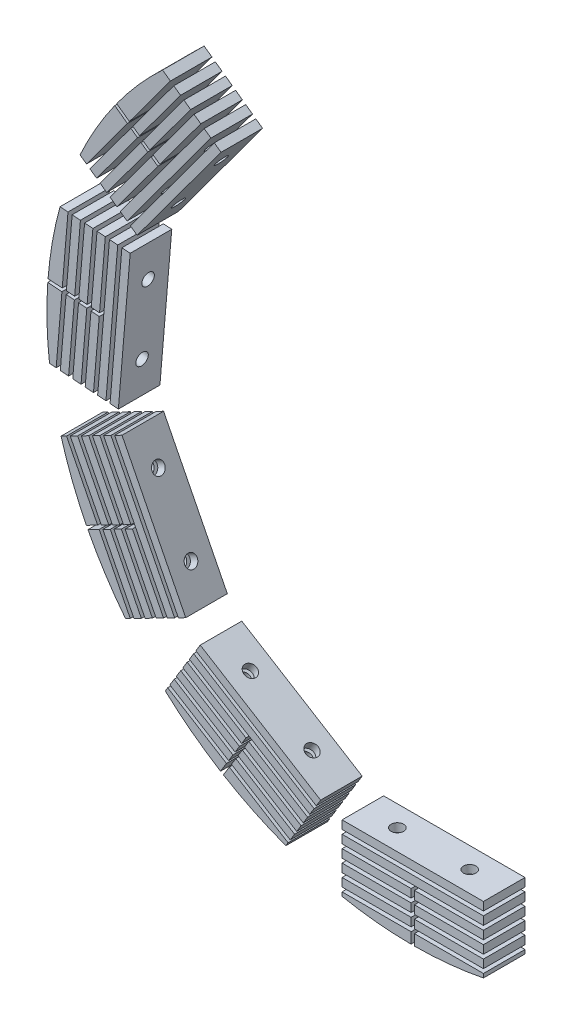
from build123d import *

# Parameters (mm, degrees)
EXTRUDE_1_DEPTH      = 25
EXTRUDE_1_2_DEPTH    = 25
EXTRUDE_1_3_DEPTH    = 25
EXTRUDE_1_4_DEPTH    = 25
EXTRUDE_1_5_DEPTH    = 25
EXTRUDE_1_6_DEPTH    = 25
EXTRUDE_1_7_DEPTH    = 25
EXTRUDE_1_8_DEPTH    = 25
EXTRUDE_1_9_DEPTH    = 25
EXTRUDE_1_10_DEPTH   = 25
SKETCH_3_W           = 195
SKETCH_3_H           = 5
CUT_EXTRUDE_2_DEPTH  = 50
SKETCH_9_R           = 7.5
CUT_EXTRUDE_5_DEPTH  = 25
SKETCH_10_R          = 7.5
CUT_EXTRUDE_6_DEPTH  = 25
SKETCH_11_R          = 7.5
CUT_EXTRUDE_7_DEPTH  = 25
SKETCH_12_R          = 7.5
CUT_EXTRUDE_8_DEPTH  = 25
SKETCH_13_R          = 7.5
CUT_EXTRUDE_9_DEPTH  = 25
SKETCH_15_W          = 182.108507318
SKETCH_15_H          = 36.421701464
CUT_EXTRUDE_13_DEPTH = 146
SKETCH_16_R          = 12.379446908
SKETCH_16_R_2        = 10.572142033
SKETCH_16_R_3        = 6.534828031
SKETCH_16_R_4        = 5.127216656
CUT_EXTRUDE_14_DEPTH = 146
SKETCH_17_W          = 4
SKETCH_17_H          = 10
EXTRUDE_2_DEPTH      = 50


with BuildPart() as part:
    # 草图2 → 凸台-拉伸1 (new, symmetric)
    with BuildSketch(Plane.XY):
        with BuildLine():
            Line((-85, -337), (-85, -431.711709362))
            ThreePointArc((-85, -431.711709362), (-43.69674025, -437.824844991), (-2, -439.995454522))
            Line((-2, -439.995454522), (-2, -337))
            Line((-2, -337), (-85, -337))
        make_face()
    extrude(amount=EXTRUDE_1_DEPTH, both=True)


with BuildPart() as body_2:
    # 草图2 → Extrude 1 2 (new, symmetric)
    with BuildSketch(Plane.XY):
        with BuildLine():
            Line((85, -337), (85, -431.711709362))
            ThreePointArc((85, -431.711709362), (43.69674025, -437.824844991), (2, -439.995454522))
            Line((2, -439.995454522), (2, -337))
            Line((2, -337), (85, -337))
        make_face()
    extrude(amount=EXTRUDE_1_2_DEPTH, both=True)


with BuildPart() as body_3:
    # 草图2 → Extrude 1 3 (new, symmetric)
    with BuildSketch(Plane.XY):
        with BuildLine():
            Line((-248.253388478, -243.237034823), (-177.430245302, -286.516156703))
            Line((-177.430245302, -286.516156703), (-231.135701078, -374.401238896))
            ThreePointArc((-231.135701078, -374.401238896), (-265.583317105, -350.806929344), (-297.639407911, -324.053672805))
            Line((-297.639407911, -324.053672805), (-248.253388478, -243.237034823))
        make_face()
    extrude(amount=EXTRUDE_1_3_DEPTH, both=True)


with BuildPart() as body_4:
    # 草图2 → Extrude 1 4 (new, symmetric)
    with BuildSketch(Plane.XY):
        with BuildLine():
            Line((-174.017081776, -288.601897517), (-227.722537551, -376.48697971))
            ThreePointArc((-227.722537551, -376.48697971), (-191.01125708, -396.376966622), (-152.579958034, -412.697657379))
            Line((-152.579958034, -412.697657379), (-103.1939386, -331.881019397))
            Line((-103.1939386, -331.881019397), (-174.017081776, -288.601897517))
        make_face()
    extrude(amount=EXTRUDE_1_4_DEPTH, both=True)


with BuildPart() as body_5:
    # 草图2 → Extrude 1 5 (new, symmetric)
    with BuildSketch(Plane.XY):
        with BuildLine():
            Line((-338.664705444, -78.103887779), (-300.799220884, -151.96324791))
            Line((-300.799220884, -151.96324791), (-392.451972299, -198.950871922))
            ThreePointArc((-392.451972299, -198.950871922), (-409.542905348, -160.855863054), (-422.94598557, -121.312378966))
            Line((-422.94598557, -121.312378966), (-338.664705444, -78.103887779))
        make_face()
    extrude(amount=EXTRUDE_1_5_DEPTH, both=True)


with BuildPart() as body_6:
    # 草图2 → Extrude 1 6 (new, symmetric)
    with BuildSketch(Plane.XY):
        with BuildLine():
            Line((-298.974378255, -155.522735146), (-390.62712967, -202.510359157))
            ThreePointArc((-390.62712967, -202.510359157), (-369.673068161, -238.624857624), (-345.39017382, -272.590586464))
            Line((-345.39017382, -272.590586464), (-261.108893694, -229.382095277))
            Line((-261.108893694, -229.382095277), (-298.974378255, -155.522735146))
        make_face()
    extrude(amount=EXTRUDE_1_6_DEPTH, both=True)


with BuildPart() as body_7:
    # 草图2 → Extrude 1 7 (new, symmetric)
    with BuildSketch(Plane.XY):
        with BuildLine():
            Line((-329.705621695, 109.946364299), (-335.908219463, 27.178449133))
            Line((-335.908219463, 27.178449133), (-438.615677805, 34.875309088))
            ThreePointArc((-438.615677805, 34.875309088), (-433.335136437, 76.293246942), (-424.152497908, 117.024179203))
            Line((-424.152497908, 117.024179203), (-329.705621695, 109.946364299))
        make_face()
    extrude(amount=EXTRUDE_1_7_DEPTH, both=True)


with BuildPart() as body_8:
    # 草图2 → Extrude 1 8 (new, symmetric)
    with BuildSketch(Plane.XY):
        with BuildLine():
            Line((-336.207139837, 23.189633944), (-438.914598179, 30.8864939))
            ThreePointArc((-438.914598179, 30.8864939), (-439.866059414, -10.855863661), (-436.856613818, -52.500466317))
            Line((-436.856613818, -52.500466317), (-342.409737605, -59.578281222))
            Line((-342.409737605, -59.578281222), (-336.207139837, 23.189633944))
        make_face()
    extrude(amount=EXTRUDE_1_8_DEPTH, both=True)


with BuildPart() as body_9:
    # 草图2 → Extrude 1 9 (new, symmetric)
    with BuildSketch(Plane.XY):
        with BuildLine():
            Line((-224.004895786, 265.736348029), (-272.455620582, 198.345493555))
            Line((-272.455620582, 198.345493555), (-356.081544524, 258.468438401))
            ThreePointArc((-356.081544524, 258.468438401), (-329.978935877, 291.056526946), (-300.904932203, 321.023709055))
            Line((-300.904932203, 321.023709055), (-224.004895786, 265.736348029))
        make_face()
    extrude(amount=EXTRUDE_1_9_DEPTH, both=True)


with BuildPart() as body_10:
    # 草图2 → Extrude 1 10 (new, symmetric)
    with BuildSketch(Plane.XY):
        with BuildLine():
            Line((-274.790595271, 195.097741532), (-358.416519213, 255.220686378))
            ThreePointArc((-358.416519213, 255.220686378), (-380.994327113, 220.098438676), (-400.141356483, 182.994248084))
            Line((-400.141356483, 182.994248084), (-323.241320066, 127.706887057))
            Line((-323.241320066, 127.706887057), (-274.790595271, 195.097741532))
        make_face()
    extrude(amount=EXTRUDE_1_10_DEPTH, both=True)


with BuildPart() as cut_extrude_2_tool:
    # 草图3 → 切除-拉伸2 (new body)
    with BuildSketch(Plane.XY.offset(25)):
        with Locations((8.886936661, -349.5)):
            Rectangle(SKETCH_3_W, SKETCH_3_H)
        with Locations((8.886936661, -364.5)):
            Rectangle(SKETCH_3_W, SKETCH_3_H)
        with Locations((8.886936661, -379.5)):
            Rectangle(SKETCH_3_W, SKETCH_3_H)
        with Locations((8.886936661, -394.5)):
            Rectangle(SKETCH_3_W, SKETCH_3_H)
        with Locations((8.886936661, -409.5)):
            Rectangle(SKETCH_3_W, SKETCH_3_H)
        with Locations((8.886936661, -424.5)):
            Rectangle(SKETCH_3_W, SKETCH_3_H)
        Polygon((-297.291118916, -317.703069409), (-131.204366758, -419.880321073), (-128.584437228, -415.621686403), (-294.671189386, -313.444434738), align=None)
        Polygon((-289.431330326, -304.927165397), (-123.344578168, -407.104417061), (-120.724648639, -402.84578239), (-286.811400796, -300.668530726), align=None)
        Polygon((-281.571541737, -292.151261385), (-115.484789579, -394.328513049), (-112.864860049, -390.069878378), (-278.951612207, -287.892626714), align=None)
        Polygon((-273.711753147, -279.375357373), (-107.625000989, -381.552609037), (-105.005071459, -377.293974366), (-271.091823617, -275.116722702), align=None)
        Polygon((-265.851964558, -266.599453361), (-99.7652124, -368.776705025), (-97.14528287, -364.518070354), (-263.232035028, -262.34081869), align=None)
        Polygon((-257.992175968, -253.823549348), (-91.90542381, -356.000801013), (-89.28549428, -351.742166342), (-255.372246438, -249.564914678), align=None)
        Polygon((-417.75778822, -115.267569798), (-329.836667785, -289.321804397), (-325.373738693, -287.067416693), (-413.294859127, -113.013182095), align=None)
        Polygon((-404.369000943, -108.504406688), (-316.447880508, -282.558641286), (-311.984951416, -280.304253583), (-399.906071851, -106.250018985), align=None)
        Polygon((-390.980213666, -101.741243578), (-303.059093232, -275.795478176), (-298.596164139, -273.541090472), (-386.517284574, -99.486855874), align=None)
        Polygon((-377.591426389, -94.978080467), (-289.670305955, -269.032315066), (-285.207376863, -266.777927362), (-373.128497297, -92.723692764), align=None)
        Polygon((-364.202639112, -88.214917357), (-276.281518678, -262.269151955), (-271.818589586, -260.014764252), (-359.73971002, -85.960529654), align=None)
        Polygon((-350.813851836, -81.451754247), (-262.892731401, -255.505988845), (-258.429802309, -253.251601141), (-346.350922743, -79.197366543), align=None)
        Polygon((-414.289146468, 120.275034501), (-430.606325918, -74.041073053), (-425.623861622, -74.459462269), (-409.306682172, 119.856645284), align=None)
        Polygon((-399.341753579, 119.019866851), (-415.658933029, -75.296240703), (-410.676468733, -75.714629919), (-394.359289283, 118.601477634), align=None)
        Polygon((-384.394360691, 117.764699201), (-400.71154014, -76.551408352), (-395.729075844, -76.969797569), (-379.411896394, 117.346309984), align=None)
        Polygon((-369.446967802, 116.509531551), (-385.764147252, -77.806576002), (-380.781682955, -78.224965219), (-364.464503506, 116.091142335), align=None)
        Polygon((-354.499574913, 115.254363901), (-370.816754363, -79.061743652), (-365.834290067, -79.480132869), (-349.517110617, 114.835974685), align=None)
        Polygon((-339.552182024, 113.999196251), (-355.869361474, -80.316911302), (-350.886897178, -80.735300519), (-334.569717728, 113.580807035), align=None)
        Polygon((-287.913805955, 319.075495331), (-403.630488843, 162.121204846), (-399.606019856, 159.154110413), (-283.889336968, 316.108400898), align=None)
        Polygon((-275.840398995, 310.174212032), (-391.557081882, 153.219921547), (-387.532612896, 150.252827114), (-271.815930008, 307.207117599), align=None)
        Polygon((-263.766992034, 301.272928732), (-379.483674922, 144.318638248), (-375.459205935, 141.351543815), (-259.742523048, 298.305834299), align=None)
        Polygon((-251.693585074, 292.371645433), (-367.410267962, 135.417354949), (-363.385798975, 132.450260516), (-247.669116087, 289.404551), align=None)
        Polygon((-239.620178114, 283.470362134), (-355.336861001, 126.51607165), (-351.312392015, 123.548977217), (-235.595709127, 280.503267701), align=None)
        Polygon((-227.546771153, 274.569078835), (-343.263454041, 117.614788351), (-339.238985054, 114.647693918), (-223.522302167, 271.601984402), align=None)
        Polygon((-76.107885054, 422.180305048), (-256.908736694, 349.132019332), (-255.035703727, 344.496100059), (-74.234852086, 417.544385775), align=None)
        Polygon((-70.488786152, 408.27254723), (-251.289637793, 335.224261513), (-249.416604826, 330.588342241), (-68.615753185, 403.636627957), align=None)
        Polygon((-64.869687251, 394.364789411), (-245.670538892, 321.316503695), (-243.797505924, 316.680584422), (-62.996654284, 389.728870138), align=None)
        Polygon((-59.25058835, 380.457031593), (-240.05143999, 307.408745876), (-238.178407023, 302.772826604), (-57.377555383, 375.82111232), align=None)
        Polygon((-53.631489449, 366.549273774), (-234.432341089, 293.500988058), (-232.559308122, 288.865068785), (-51.758456481, 361.913354501), align=None)
        Polygon((-48.012390547, 352.641515956), (-228.813242188, 279.593230239), (-226.940209221, 274.957310967), (-46.13935758, 348.005596683), align=None)
    extrude(amount=-CUT_EXTRUDE_2_DEPTH)


with BuildPart() as part_1:
    add(part.part)

    # 切除-拉伸2: cut by cut_extrude_2_tool
    add(cut_extrude_2_tool.part, mode=Mode.SUBTRACT)


with BuildPart() as body_2_1:
    add(body_2.part)

    # 切除-拉伸2: cut by cut_extrude_2_tool
    add(cut_extrude_2_tool.part, mode=Mode.SUBTRACT)


with BuildPart() as body_3_1:
    add(body_3.part)

    # 切除-拉伸2: cut by cut_extrude_2_tool
    add(cut_extrude_2_tool.part, mode=Mode.SUBTRACT)


with BuildPart() as body_4_1:
    add(body_4.part)

    # 切除-拉伸2: cut by cut_extrude_2_tool
    add(cut_extrude_2_tool.part, mode=Mode.SUBTRACT)


with BuildPart() as body_5_1:
    add(body_5.part)

    # 切除-拉伸2: cut by cut_extrude_2_tool
    add(cut_extrude_2_tool.part, mode=Mode.SUBTRACT)


with BuildPart() as body_6_1:
    add(body_6.part)

    # 切除-拉伸2: cut by cut_extrude_2_tool
    add(cut_extrude_2_tool.part, mode=Mode.SUBTRACT)


with BuildPart() as body_7_1:
    add(body_7.part)

    # 切除-拉伸2: cut by cut_extrude_2_tool
    add(cut_extrude_2_tool.part, mode=Mode.SUBTRACT)


with BuildPart() as body_8_1:
    add(body_8.part)

    # 切除-拉伸2: cut by cut_extrude_2_tool
    add(cut_extrude_2_tool.part, mode=Mode.SUBTRACT)


with BuildPart() as body_9_1:
    add(body_9.part)

    # 切除-拉伸2: cut by cut_extrude_2_tool
    add(cut_extrude_2_tool.part, mode=Mode.SUBTRACT)


with BuildPart() as body_10_1:
    add(body_10.part)

    # 切除-拉伸2: cut by cut_extrude_2_tool
    add(cut_extrude_2_tool.part, mode=Mode.SUBTRACT)


with BuildPart() as cut_extrude_5_tool:
    # 草图9 → 切除-拉伸5 (new body)
    with BuildSketch(Plane(origin=(0, -352, 0), x_dir=(1, 0, 0), z_dir=(0, 1, 0))):
        with Locations(Location((43.5, 0, 0), (0, 0, 180))):
            Circle(SKETCH_9_R)
        with Locations((-43.5, 0)):
            Circle(SKETCH_9_R)
    extrude(amount=-CUT_EXTRUDE_5_DEPTH)


with BuildPart() as part_2:
    add(part_1.part)

    # 切除-拉伸5: cut by cut_extrude_5_tool
    add(cut_extrude_5_tool.part, mode=Mode.SUBTRACT)


with BuildPart() as body_2_2:
    add(body_2_1.part)

    # 切除-拉伸5: cut by cut_extrude_5_tool
    add(cut_extrude_5_tool.part, mode=Mode.SUBTRACT)


with BuildPart() as cut_extrude_6_tool:
    # 草图10 → 切除-拉伸6 (new body)
    with BuildSketch(Plane(origin=(-184.114299344, -299.273522294, 0), x_dir=(0.8517269341430569, -0.5239859059700643, 0), z_dir=(0.5239859059700643, 0.8517269341430569, 0))):
        with Locations(Location((44.551502258, 0, 0), (0, 0, 180))):
            Circle(SKETCH_10_R)
        with Locations(Location((-42.491505156, 0, 0), (0, 0, 180))):
            Circle(SKETCH_10_R)
    extrude(amount=-CUT_EXTRUDE_6_DEPTH)


with BuildPart() as body_3_2:
    add(body_3_1.part)

    # 切除-拉伸6: cut by cut_extrude_6_tool
    add(cut_extrude_6_tool.part, mode=Mode.SUBTRACT)


with BuildPart() as body_4_2:
    add(body_4_1.part)

    # 切除-拉伸6: cut by cut_extrude_6_tool
    add(cut_extrude_6_tool.part, mode=Mode.SUBTRACT)


with BuildPart() as cut_extrude_7_tool:
    # 草图11 → 切除-拉伸7 (new body)
    with BuildSketch(Plane(origin=(-312.276714487, -157.742319149, 0), x_dir=(0, 0, -1), z_dir=(0.8925858184521096, 0.4508775406894622, 0))):
        with Locations(Location((0, 41.40721903, 0), (0, 0, 90))):
            Circle(SKETCH_11_R)
        with Locations(Location((0, -45.594338645, 0), (0, 0, 90))):
            Circle(SKETCH_11_R)
    extrude(amount=-CUT_EXTRUDE_7_DEPTH)


with BuildPart() as body_5_2:
    add(body_5_1.part)

    # 切除-拉伸7: cut by cut_extrude_7_tool
    add(cut_extrude_7_tool.part, mode=Mode.SUBTRACT)


with BuildPart() as body_6_2:
    add(body_6_1.part)

    # 切除-拉伸7: cut by cut_extrude_7_tool
    add(cut_extrude_7_tool.part, mode=Mode.SUBTRACT)


with BuildPart() as cut_extrude_8_tool:
    # 草图12 → 切除-拉伸8 (new body)
    with BuildSketch(Plane(origin=(-346.680395482, 29.11156618, 0), x_dir=(0, 0, -1), z_dir=(0.9964928592495088, -0.08367784333226239, 0))):
        with Locations(Location((0, -46.624584154, 0), (0, 0, 90))):
            Circle(SKETCH_12_R)
        with Locations(Location((0, 40.37892068, 0), (0, 0, 90))):
            Circle(SKETCH_12_R)
    extrude(amount=-CUT_EXTRUDE_8_DEPTH)


with BuildPart() as body_7_2:
    add(body_7_1.part)

    # 切除-拉伸8: cut by cut_extrude_8_tool
    add(cut_extrude_8_tool.part, mode=Mode.SUBTRACT)


with BuildPart() as body_8_2:
    add(body_8_1.part)

    # 切除-拉伸8: cut by cut_extrude_8_tool
    add(cut_extrude_8_tool.part, mode=Mode.SUBTRACT)


with BuildPart() as cut_extrude_9_tool:
    # 草图13 → 切除-拉伸9 (new body)
    with BuildSketch(Plane(origin=(-278.562041532, 205.373649392, 0), x_dir=(0, 0, -1), z_dir=(0.8048937973559566, -0.593418886603644, 0))):
        with Locations(Location((0, -47.645254375, 0), (0, 0, 90))):
            Circle(SKETCH_13_R)
        with Locations(Location((0, 39.360976604, 0), (0, 0, 90))):
            Circle(SKETCH_13_R)
    extrude(amount=-CUT_EXTRUDE_9_DEPTH)


with BuildPart() as body_9_2:
    add(body_9_1.part)

    # 切除-拉伸9: cut by cut_extrude_9_tool
    add(cut_extrude_9_tool.part, mode=Mode.SUBTRACT)


with BuildPart() as body_10_2:
    add(body_10_1.part)

    # 切除-拉伸9: cut by cut_extrude_9_tool
    add(cut_extrude_9_tool.part, mode=Mode.SUBTRACT)


with BuildPart() as cut_extrude_13_tool:
    # 草图15 → 切除-拉伸13 (new body)
    with BuildSketch(Plane(origin=(0, 0, -25), x_dir=(-1, 0, 0), z_dir=(0, 0, -1))):
        Polygon((95.824271396, -320.042426741), (108.214571248, -340.096920493), (253.008798153, -251.018917764), (243.902808303, -236.217342514), align=None)
        Polygon((278.147006967, 197.510837206), (226.515866252, 267.541612852), (203.864456535, 253.857614626), (290.435206143, 110.555234253), (327.404302132, 130.699867336), align=None)
        with Locations((-0.496379734, -332.061186913)):
            Rectangle(SKETCH_15_W, SKETCH_15_H)
        Polygon((341.788125028, 27.619087139), (349.068390675, -59.079284158), (334.356354276, -60.314688371), (320.130547839, 109.095922209), (334.842584239, 110.331326423), align=None)
        Polygon((305.981565456, -159.115110416), (268.558059549, -233.201059781), (242.774738531, -220.176967161), (319.425292799, -68.434661231), (345.208613817, -81.458753852), align=None)
    extrude(amount=-CUT_EXTRUDE_13_DEPTH)


with BuildPart() as part_3:
    add(part_2.part)

    # 切除-拉伸13: cut by cut_extrude_13_tool
    add(cut_extrude_13_tool.part, mode=Mode.SUBTRACT)



with BuildPart() as body_2_3:
    add(body_2_2.part)

    # 切除-拉伸13: cut by cut_extrude_13_tool
    add(cut_extrude_13_tool.part, mode=Mode.SUBTRACT)


with BuildPart() as body_3_3:
    add(body_3_2.part)

    # 切除-拉伸13: cut by cut_extrude_13_tool
    add(cut_extrude_13_tool.part, mode=Mode.SUBTRACT)


with BuildPart() as body_4_3:
    add(body_4_2.part)

    # 切除-拉伸13: cut by cut_extrude_13_tool
    add(cut_extrude_13_tool.part, mode=Mode.SUBTRACT)


with BuildPart() as body_5_3:
    add(body_5_2.part)

    # 切除-拉伸13: cut by cut_extrude_13_tool
    add(cut_extrude_13_tool.part, mode=Mode.SUBTRACT)


with BuildPart() as body_6_3:
    add(body_6_2.part)

    # 切除-拉伸13: cut by cut_extrude_13_tool
    add(cut_extrude_13_tool.part, mode=Mode.SUBTRACT)


with BuildPart() as body_7_3:
    add(body_7_2.part)

    # 切除-拉伸13: cut by cut_extrude_13_tool
    add(cut_extrude_13_tool.part, mode=Mode.SUBTRACT)


with BuildPart() as body_8_3:
    add(body_8_2.part)

    # 切除-拉伸13: cut by cut_extrude_13_tool
    add(cut_extrude_13_tool.part, mode=Mode.SUBTRACT)


with BuildPart() as body_9_3:
    add(body_9_2.part)

    # 切除-拉伸13: cut by cut_extrude_13_tool
    add(cut_extrude_13_tool.part, mode=Mode.SUBTRACT)


with BuildPart() as body_10_3:
    add(body_10_2.part)

    # 切除-拉伸13: cut by cut_extrude_13_tool
    add(cut_extrude_13_tool.part, mode=Mode.SUBTRACT)


with BuildPart() as cut_extrude_14_tool:
    # 草图16 → 切除-拉伸14 (new body)
    with BuildSketch(Plane(origin=(0, 0, -25), x_dir=(-1, 0, 0), z_dir=(0, 0, -1))):
        with Locations((248.253388478, -243.237034823)):
            Circle(SKETCH_16_R)
        with Locations((337.506728105, -76.937031464)):
            Circle(SKETCH_16_R_2)
        with Locations((329.705621695, 109.946364299)):
            Circle(SKETCH_16_R_3)
        with Locations((323.241320066, 127.706887057)):
            Circle(SKETCH_16_R_4)
    extrude(amount=-CUT_EXTRUDE_14_DEPTH)


with BuildPart() as body_3_4:
    add(body_3_3.part)

    # 切除-拉伸14: cut by cut_extrude_14_tool
    add(cut_extrude_14_tool.part, mode=Mode.SUBTRACT)


with BuildPart() as body_5_4:
    add(body_5_3.part)

    # 切除-拉伸14: cut by cut_extrude_14_tool
    add(cut_extrude_14_tool.part, mode=Mode.SUBTRACT)


with BuildPart() as body_7_4:
    add(body_7_3.part)

    # 切除-拉伸14: cut by cut_extrude_14_tool
    add(cut_extrude_14_tool.part, mode=Mode.SUBTRACT)


with BuildPart() as body_10_4:
    add(body_10_3.part)

    # 切除-拉伸14: cut by cut_extrude_14_tool
    add(cut_extrude_14_tool.part, mode=Mode.SUBTRACT)


with BuildPart() as part_4:
    add(part_3.part)

    add(body_2_3.part)  # 凸台-拉伸2 merges body 2

    add(body_3_4.part)  # 凸台-拉伸2 merges body 3

    add(body_4_3.part)  # 凸台-拉伸2 merges body 4

    add(body_5_4.part)  # 凸台-拉伸2 merges body 5

    add(body_6_3.part)  # 凸台-拉伸2 merges body 6

    add(body_7_4.part)  # 凸台-拉伸2 merges body 7

    add(body_8_3.part)  # 凸台-拉伸2 merges body 8

    add(body_9_3.part)  # 凸台-拉伸2 merges body 9

    add(body_10_4.part)  # 凸台-拉伸2 merges body 10
    # 草图17 → 凸台-拉伸2 (add)
    with BuildSketch(Plane(origin=(0, 0, -25), x_dir=(-1, 0, 0), z_dir=(0, 0, -1))):
        with Locations((0, -357)):
            Rectangle(SKETCH_17_W, SKETCH_17_H)
        with Locations((0, -372)):
            Rectangle(SKETCH_17_W, SKETCH_17_H)
        Polygon((190.136709254, -307.309363141), (184.92233388, -298.776416131), (181.515410894, -300.872369136), (186.729786268, -309.405316146), align=None)
        Polygon((189.336973954, -313.671789651), (194.551349328, -322.204736661), (197.958272314, -320.108783655), (192.74389694, -311.575836646), align=None)
        Polygon((323.779320283, -168.239486925), (332.678197697, -172.80167518), (334.48174015, -169.231267982), (325.582862737, -164.669079727), align=None)
        Polygon((321.13342403, -162.3879856), (312.234546616, -157.825797345), (310.431004163, -161.396204543), (319.329881577, -165.958392798), align=None)
        Polygon((371.705444128, 29.861080263), (361.733004428, 29.113749222), (362.067729286, 25.127617208), (372.040168985, 25.874948249), align=None)
        Polygon((356.746784578, 28.740083701), (346.774344878, 27.99275266), (347.109069736, 24.006620646), (357.081509436, 24.753951688), align=None)
        Polygon((287.953103773, 209.487425186), (279.833142203, 203.649570384), (282.206987753, 200.429764607), (290.326949324, 206.267619409), align=None)
        Polygon((300.13304613, 218.244207389), (292.013084559, 212.406352587), (294.386930109, 209.18654681), (302.50689168, 215.024401612), align=None)
    extrude(amount=-EXTRUDE_2_DEPTH)


solid = part_4.part
